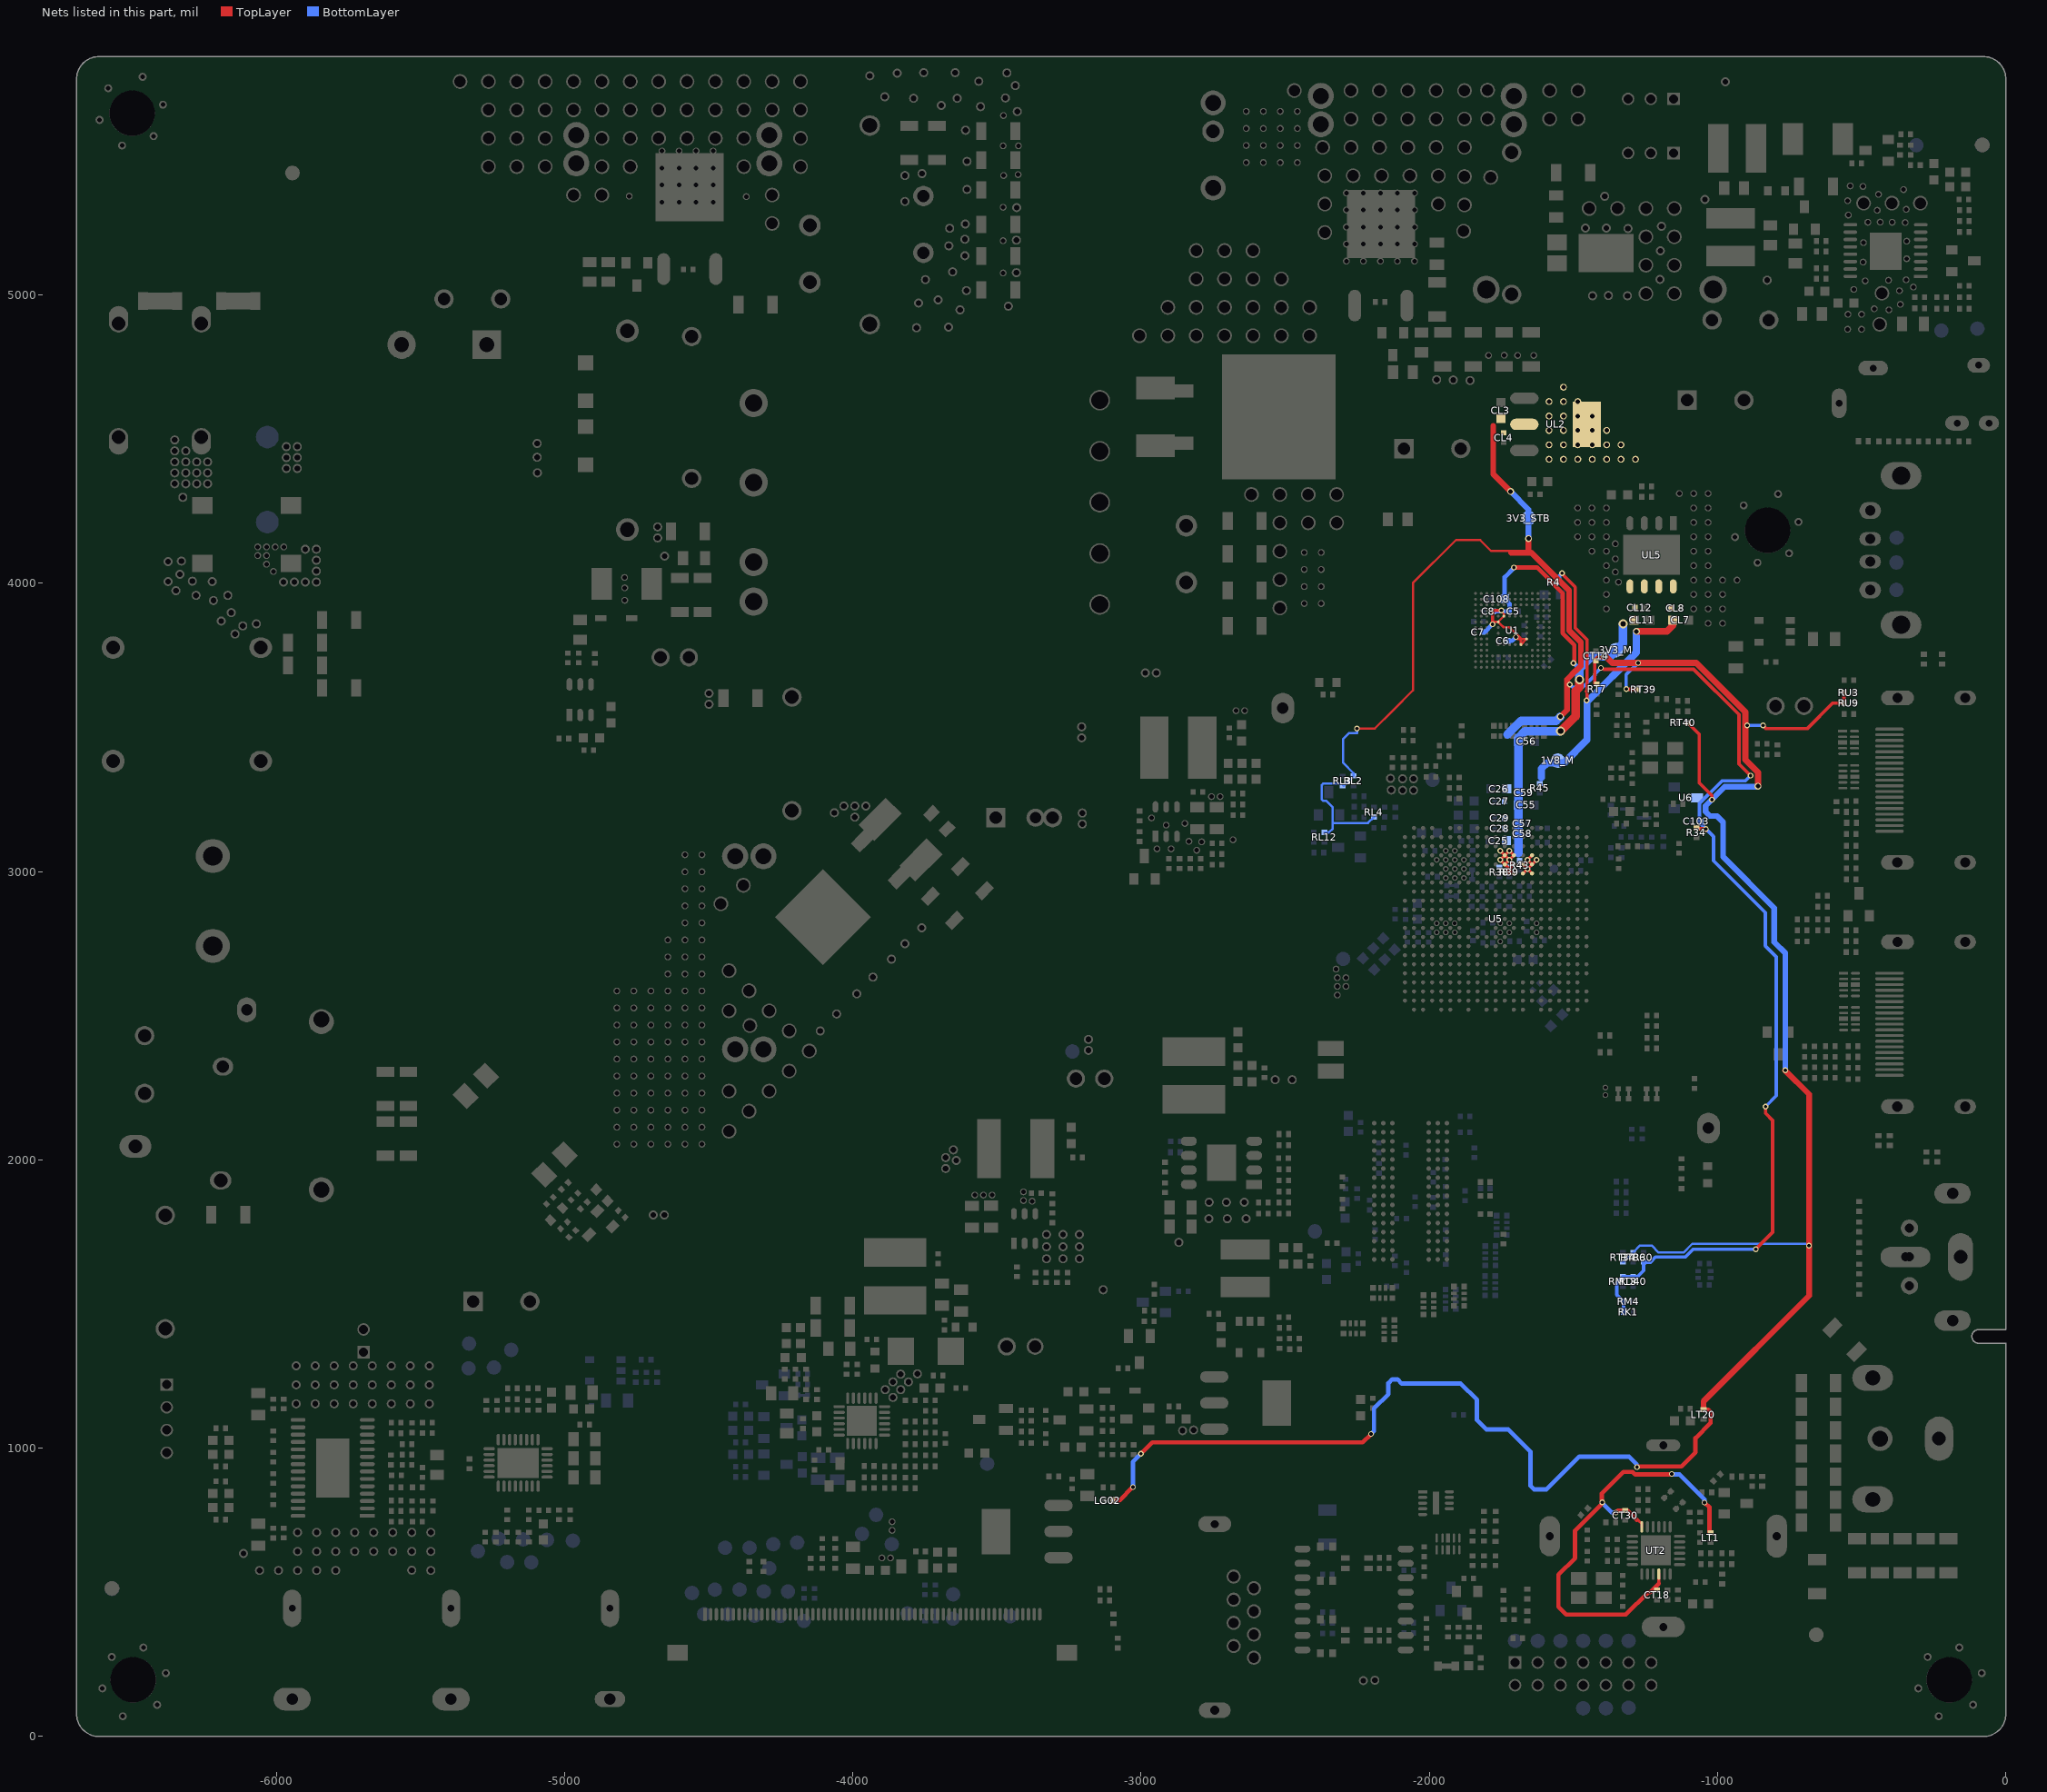
[diagram p0: the nets of this part, all layers, seen from the top]
# Altium PCB MISC84395.PcbDoc (part 8 of 26)
Units mil, origin at the board's own origin, x right, y up, seen from the top; angles counter-clockwise.
Board outline 6692.91 x 5826.77 mil, 2 copper layers (TopLayer, BottomLayer), stack 61.855 mil thick; 951 components, 565 nets, 4374 pads, 1804 vias.
Unrouted connection lines stored in the file: 1.

## Free pads (board coordinates)
  round 157.48 on Keep-Out: 0(-13188.98,196.85) 0(-6305.12,5435.04) 0(-196.85,5629.92) 1(-391.73,393.7)
  oval 196.85x157.48 on Keep-Out: 0(-12395.74,5629.92) 0(-990.09,196.85)
  round 47.24 on Bottom Solder: 0(-6402,5173)
  round 31.5 hole 19.68 paste-15.75 mask-15.75: VIA5(-6375,4006) VIA5(-6375,4075) VIA5(-6352,4345) VIA5(-6352,4383) VIA5(-6352,4421) VIA5(-6352,4459) VIA5(-6352,4497) VIA5(-6348,3974) VIA5(-6334,4031) VIA5(-6329,4077) VIA5(-6324,4298) VIA5(-6314,4345) VIA5(-6314,4383) VIA5(-6314,4421) VIA5(-6314,4459) VIA5(-6291,4007) VIA5(-6278,3958) VIA5(-6276,4345) VIA5(-6276,4383) VIA5(-6276,4421) VIA5(-6238,4345) VIA5(-6238,4383) VIA5(-6238,4421) VIA5(-6222,4006) VIA5(-6218,3940) VIA5(-6191,3869) VIA5(-6168,3958) VIA5(-6156,3898) VIA5(-6143,3824) VIA5(-6116,3852) VIA5(-6113.94,635) VIA5(-6069,3859) VIA5(-6057.94,576) VIA5(-5991.94,576) VIA5(-5975,4004) VIA5(-5965,4398) VIA5(-5965,4436) VIA5(-5965,4474) VIA5(-5937,4004) VIA5(-5930.94,1286) VIA5(-5930.94,1220) VIA5(-5930.94,1154) VIA5(-5927,4398) VIA5(-5927,4436) VIA5(-5927,4474) VIA5(-5925.94,576) VIA5(-5925.94,642) VIA5(-5925.94,708) VIA5(-5899,4004) VIA5(-5899,4118) VIA5(-5864.94,1286) VIA5(-5864.94,1154) VIA5(-5864.94,1220) VIA5(-5861,4004) VIA5(-5861,4042) VIA5(-5861,4080) VIA5(-5861,4118) VIA5(-5859.94,576) VIA5(-5859.94,642) VIA5(-5859.94,708) VIA5(-5798.94,1286) VIA5(-5798.94,1220) VIA5(-5798.94,1154) VIA5(-5793.94,576) VIA5(-5793.94,642) VIA5(-5793.94,708) VIA5(-5732.94,1286) VIA5(-5732.94,1154) VIA5(-5732.94,1220) VIA5(-5727.94,642) VIA5(-5727.94,708) VIA5(-5666.95,1286) VIA5(-5666.94,1154) VIA5(-5666.94,1220) VIA5(-5661.94,642) VIA5(-5661.94,708) VIA5(-5600.95,1286) VIA5(-5600.95,1154) VIA5(-5600.95,1220) VIA5(-5595.94,642) VIA5(-5595.94,708) VIA5(-5534.95,1286) VIA5(-5534.95,1154) VIA5(-5534.95,1220) VIA5(-5530,577) VIA5(-5529.94,642) VIA5(-5529.94,708) VIA5(-5468.95,1286) VIA5(-5468.95,1154) VIA5(-5468.95,1220) VIA5(-5463.94,576) VIA5(-5463.94,642) VIA5(-5463.94,708) VIA5(-5095.08,4437) VIA5(-5095.08,4485) VIA5(-5094,4383) VIA5(-4692,1809) VIA5(-4677,4157.3) VIA5(-4677,4195.3) VIA5(-4654,1809) VIA5(-4653,4094.3) VIA5(-4499,3580) VIA5(-4499,3618) VIA5(-4113,2447) VIA5(-4064,3204) VIA5(-4056,2506) VIA5(-4031,3227) VIA5(-3993,3189) VIA5(-3993,3227) VIA5(-3986,2576) VIA5(-3955,3227) VIA5(-3941,5760) VIA5(-3930,2634) VIA5(-3889,5687) VIA5(-3887.61,1203.13) VIA5(-3866,2696) VIA5(-3860.74,1176.26) VIA5(-3860.74,1230) VIA5(-3846,5769) VIA5(-3833.87,1203.13) VIA5(-3833.87,1256.87) VIA5(-3819,2750) VIA5(-3819,5324) VIA5(-3819,5414) VIA5(-3807,1230) VIA5(-3789,5682) VIA5(-3779,4886) VIA5(-3776,1258) VIA5(-3772,4972) VIA5(-3761,2805) VIA5(-3760,5421) VIA5(-3754,5771) VIA5(-3748,5053) VIA5(-3704,4983) VIA5(-3693,5657) VIA5(-3677.87,1970.13) VIA5(-3677.87,2008.13) VIA5(-3668,4888) VIA5(-3667,5170) VIA5(-3664,5231) VIA5(-3654,5080) VIA5(-3651,2035) VIA5(-3645,5771) VIA5(-3641.13,1998.13) VIA5(-3638,5682) VIA5(-3628,4948) VIA5(-3611,5136) VIA5(-3611,5193) VIA5(-3610,5246) VIA5(-3609,5571) VIA5(-3606,5015) VIA5(-3604,5366) VIA5(-3604,5463) VIA5(-3563,5741) VIA5(-3557,5653) VIA5(-3470.56,5683) VIA5(-3465.56,5770) VIA5(-3460.56,4961) VIA5(-3436.56,5726) VIA5(-3432.56,5077) VIA5(-3432.56,5190) VIA5(-3431.56,5303) VIA5(-3429.56,5636) VIA5(-3328,1657) VIA5(-3328,1699) VIA5(-3328,1741) VIA5(-3271,1657) VIA5(-3271,1699) VIA5(-3271,1741) VIA5(-3214,1657) VIA5(-3214,1699) VIA5(-3214,1741) VIA5(-3206,3464) VIA5(-3206,3502) VIA5(-3204,3165) VIA5(-3204,3203) VIA5(-3182.5,2380) VIA5(-3182.5,2418) VIA5(-3131.42,1549.58) VIA5(-2985.23,3688.77) VIA5(-2947.23,3688.77) VIA5(-2869,1714) VIA5(-2856,1061) VIA5(-2818,1063) VIA5(-2765,1796) VIA5(-2764,1853) VIA5(-2704,1853) VIA5(-2701,1796) VIA5(-2642,1853) VIA5(-2636,1796) VIA5(-2535,2278) VIA5(-2476,2278) VIA5(-2228.87,194.13) VIA5(-2189,195) VIA5(-2135,3323) VIA5(-2132,3283) VIA5(-2093,3282) VIA5(-2093,3322) VIA5(-2055,3282) VIA5(-2055,3322) VIA5(-1975,4706) VIA5(-1917,4705) VIA5(-1859,4703) VIA5(-1458.89,5232) VIA5(-1433.89,4997) VIA5(-1391.89,5342) VIA5(-1385.89,5232) VIA5(-1378.89,4998) VIA5(-1312.89,4997) VIA5(-1310.89,5230) VIA5(-1199.89,5054) VIA5(-1198.89,5153) VIA5(-1194.89,5238) VIA5(-1044,5331) VIA5(-973,5739) VIA5(-828,5051)
  round 23.62 hole 15.75 paste-15.75 mask-15.75: VIA5(-6064,4096) VIA5(-6064,4126) VIA5(-6034,4066) VIA5(-6034,4096) VIA5(-6034,4126) VIA5(-6010,4041) VIA5(-6004,4126) VIA5(-5974,4126) VIA5(-4818.66,2054.38) VIA5(-4818.66,2113.43) VIA5(-4818.66,2172.49) VIA5(-4818.66,2231.54) VIA5(-4818.66,2290.6) VIA5(-4818.66,2349.65) VIA5(-4818.66,2408.71) VIA5(-4818.66,2467.76) VIA5(-4818.66,2526.82) VIA5(-4818.66,2585.87) VIA5(-4792,4020) VIA5(-4791,3941) VIA5(-4791,3984) VIA5(-4775.66,5342.71) VIA5(-4759.6,2054.38) VIA5(-4759.6,2113.43) VIA5(-4759.6,2172.49) VIA5(-4759.6,2231.54) VIA5(-4759.6,2290.6) VIA5(-4759.6,2349.65) VIA5(-4759.6,2408.71) VIA5(-4759.6,2467.76) VIA5(-4759.6,2526.82) VIA5(-4759.6,2585.87) VIA5(-4700.55,2054.38) VIA5(-4700.55,2113.43) VIA5(-4700.55,2172.49) VIA5(-4700.55,2231.54) VIA5(-4700.55,2290.6) VIA5(-4700.55,2349.65) VIA5(-4700.55,2408.71) VIA5(-4700.55,2467.76) VIA5(-4700.55,2526.82) VIA5(-4700.55,2585.87) VIA5(-4661.66,5321.71) VIA5(-4661.66,5380.76) VIA5(-4661.66,5439.82) VIA5(-4661.66,5498.87) VIA5(-4641.49,2054.38) VIA5(-4641.49,2113.43) VIA5(-4641.49,2172.49) VIA5(-4641.49,2231.54) VIA5(-4641.49,2290.6) VIA5(-4641.49,2349.65) VIA5(-4641.49,2408.71) VIA5(-4641.49,2467.76) VIA5(-4641.49,2526.82) VIA5(-4641.49,2585.87) VIA5(-4641.49,2644.93) VIA5(-4641.49,2703.99) VIA5(-4641.49,2763.04) VIA5(-4602.6,5321.71) VIA5(-4602.6,5380.76) VIA5(-4602.6,5439.82) VIA5(-4602.6,5498.87) VIA5(-4582.44,2054.38) VIA5(-4582.44,2113.43) VIA5(-4582.44,2172.49) VIA5(-4582.44,2231.54) VIA5(-4582.44,2290.6) VIA5(-4582.44,2349.65) VIA5(-4582.44,2408.71) VIA5(-4582.44,2467.76) VIA5(-4582.44,2526.82) VIA5(-4582.44,2585.87) VIA5(-4582.44,2644.93) VIA5(-4582.44,2703.99) VIA5(-4582.44,2763.04) VIA5(-4582.44,2822.1) VIA5(-4582.44,2881.15) VIA5(-4582.44,2940.21) VIA5(-4582.44,2999.26) VIA5(-4582.44,3058.32) VIA5(-4543.55,5321.71) VIA5(-4543.55,5380.76) VIA5(-4543.55,5439.82) VIA5(-4543.55,5498.87) VIA5(-4523.38,2054.38) VIA5(-4523.38,2113.43) VIA5(-4523.38,2172.49) VIA5(-4523.38,2231.54) VIA5(-4523.38,2290.6) VIA5(-4523.38,2349.65) VIA5(-4523.38,2408.71) VIA5(-4523.38,2467.76) VIA5(-4523.38,2526.82) VIA5(-4523.38,2585.87) VIA5(-4523.38,2644.93) VIA5(-4523.38,2703.99) VIA5(-4523.38,2763.04) VIA5(-4523.38,2822.1) VIA5(-4523.38,2881.15) VIA5(-4523.38,2940.21) VIA5(-4523.38,2999.26) VIA5(-4523.38,3058.32) VIA5(-4484.49,5321.71) VIA5(-4484.49,5380.76) VIA5(-4484.49,5439.82) VIA5(-4484.49,5498.87) VIA5(-4369.66,5340.71) VIA5(-3899,619.5) VIA5(-3869,619.5) VIA5(-3864,715) VIA5(-3864,745) VIA5(-3577,1878) VIA5(-3547,1878) VIA5(-3517,1878) VIA5(-3478.56,5076) VIA5(-3478.56,5188) VIA5(-3478.56,5304) VIA5(-3478.56,5517) VIA5(-3477.56,5622) VIA5(-3476.56,5414) VIA5(-3426.56,5417) VIA5(-3425.56,5517) VIA5(-3408,1859) VIA5(-3408,1889) VIA5(-3378,1857) VIA5(-2964,3186) VIA5(-2944.83,3078.43) VIA5(-2913,3161) VIA5(-2895.85,3078.43) VIA5(-2848,3166.69) VIA5(-2834,3105) VIA5(-2807,3074) VIA5(-2790,3103) VIA5(-2756,3260) VIA5(-2726,3260) VIA5(-2681,3110) VIA5(-2671,3558) VIA5(-2641,3558) VIA5(-2635.01,5459.37) VIA5(-2635.01,5518.43) VIA5(-2635.01,5577.48) VIA5(-2635.01,5636.54) VIA5(-2575.95,5459.37) VIA5(-2575.95,5518.43) VIA5(-2575.95,5577.48) VIA5(-2575.95,5636.54) VIA5(-2516.9,5459.37) VIA5(-2516.9,5518.43) VIA5(-2516.9,5577.48) VIA5(-2516.9,5636.54) VIA5(-2457.84,5459.37) VIA5(-2457.84,5518.43) VIA5(-2457.84,5577.48) VIA5(-2457.84,5636.54) VIA5(-2434.06,3929.43) VIA5(-2434.06,3988.48) VIA5(-2434.06,4047.54) VIA5(-2434.06,4106.59) VIA5(-2375.01,3929.43) VIA5(-2375.01,3988.48) VIA5(-2375.01,4047.54) VIA5(-2375.01,4106.59) VIA5(-2323.65,2661.74) VIA5(-2319.65,2571.74) VIA5(-2319.65,2601.74) VIA5(-2319.65,2631.74) VIA5(-2289.65,2601.74) VIA5(-2289.65,2631.74) VIA5(-2288.06,5117.37) VIA5(-2288.06,5176.43) VIA5(-2288.06,5235.48) VIA5(-2288.06,5294.54) VIA5(-2288.06,5353.59) VIA5(-2229.01,5117.37) VIA5(-2229.01,5176.43) VIA5(-2229.01,5235.48) VIA5(-2229.01,5294.54) VIA5(-2229.01,5353.59) VIA5(-2169.95,5117.37) VIA5(-2169.95,5176.43) VIA5(-2169.95,5235.48) VIA5(-2169.95,5294.54) VIA5(-2169.95,5353.59) VIA5(-2110.9,5117.37) VIA5(-2110.9,5176.43) VIA5(-2110.9,5235.48) VIA5(-2110.9,5294.54) VIA5(-2110.9,5353.59) VIA5(-2051.84,5117.37) VIA5(-2051.84,5176.43) VIA5(-2051.84,5235.48) VIA5(-2051.84,5294.54) VIA5(-2051.84,5353.59) VIA5(-1795,4790) VIA5(-1740,4791) VIA5(-1694,4790) VIA5(-1638,4790) VIA5(-1585,4430) VIA5(-1585,4480) VIA5(-1585,4530) VIA5(-1585,4580) VIA5(-1585,4630) VIA5(-1535,4430) VIA5(-1535,4480) VIA5(-1535,4530) VIA5(-1535,4580) VIA5(-1535,4630) VIA5(-1535,4680) VIA5(-1486,4161) VIA5(-1486,4211) VIA5(-1486,4261) VIA5(-1485,4430) VIA5(-1485,4480) VIA5(-1485,4530) VIA5(-1485,4580) VIA5(-1485,4630) VIA5(-1436,4111) VIA5(-1436,4161) VIA5(-1436,4211) VIA5(-1436,4261) VIA5(-1435,4430) VIA5(-1435,4480) VIA5(-1435,4530) VIA5(-1435,4580) VIA5(-1386,3911) VIA5(-1386,3961) VIA5(-1386,4011) VIA5(-1386,4061) VIA5(-1386,4111) VIA5(-1386,4161) VIA5(-1386,4211) VIA5(-1386,4261) VIA5(-1385,4430) VIA5(-1385,4480) VIA5(-1385,4530) VIA5(-1355,4039) VIA5(-1355,4084.5) VIA5(-1355,4137) VIA5(-1344,4004) VIA5(-1335,4430) VIA5(-1335,4480) VIA5(-1285,4430) VIA5(-1133.04,4311) VIA5(-1083.04,4061) VIA5(-1083.04,4111) VIA5(-1083.04,4161) VIA5(-1083.04,4211) VIA5(-1083.04,4261) VIA5(-1083.04,4311) VIA5(-1083.04,3911) VIA5(-1083.04,3961) VIA5(-1083.04,4011) VIA5(-1033.04,3861) VIA5(-1033.04,3911) VIA5(-1033.04,3961) VIA5(-1033.04,4011) VIA5(-1033.04,4061) VIA5(-1033.04,4111) VIA5(-1033.04,4161) VIA5(-1033.04,4211) VIA5(-1033.04,4261) VIA5(-1033.04,4311) VIA5(-983.04,3911) VIA5(-983.04,4011) VIA5(-983.04,3861) VIA5(-983.04,3961) VIA5(-933.04,4011) VIA5(-549.19,5326.87) VIA5(-549,4881) VIA5(-548,4933) VIA5(-546.69,5276.87) VIA5(-540,5378) VIA5(-528,5019) VIA5(-501,4881) VIA5(-501,4933) VIA5(-496,5376) VIA5(-495.19,5113.87) VIA5(-494.19,5181.37) VIA5(-488.19,5048.37) VIA5(-479.19,5251.87) VIA5(-457,4952) VIA5(-446.19,5293.37) VIA5(-442,5349) VIA5(-436.19,5252.37) VIA5(-407.19,5050.87) VIA5(-406,4948) VIA5(-394.69,5251.79) VIA5(-369.19,5014.37) VIA5(-366.19,4967.37) VIA5(-355,5365) VIA5(-349.69,5250.87) VIA5(-346.19,5052.37) VIA5(-345.69,5296.87) VIA5(-344.19,5125.37) VIA5(-344.19,5186.37) VIA5(-321,5027)
  round 51.18 hole 39.37 paste-25.59 mask-2: VIA5(-5362.49,5740.1) VIA5(-5264.06,5444.82) VIA5(-5264.06,5543.25) VIA5(-5264.06,5641.67) VIA5(-5264.06,5740.1) VIA5(-5165.64,5444.82) VIA5(-5165.64,5543.25) VIA5(-5165.64,5641.67) VIA5(-5165.64,5740.1) VIA5(-5067.21,5444.82) VIA5(-5067.21,5543.25) VIA5(-5067.21,5641.67) VIA5(-5067.21,5740.1) VIA5(-4968.79,5346.4) VIA5(-4968.79,5641.67) VIA5(-4968.79,5740.1) VIA5(-4870.36,5346.4) VIA5(-4870.36,5444.82) VIA5(-4870.36,5543.25) VIA5(-4870.36,5641.67) VIA5(-4870.36,5740.1) VIA5(-4771.94,5444.82) VIA5(-4771.94,5543.25) VIA5(-4771.94,5641.67) VIA5(-4771.94,5740.1) VIA5(-4673.51,5543.25) VIA5(-4673.51,5641.67) VIA5(-4673.51,5740.1) VIA5(-4575.09,5543.25) VIA5(-4575.09,5641.67) VIA5(-4575.09,5740.1) VIA5(-4476.66,5543.25) VIA5(-4476.66,5641.67) VIA5(-4476.66,5740.1) VIA5(-4457.6,2888.4) VIA5(-4429.38,2517.02) VIA5(-4429.38,2656.21) VIA5(-4429.37,2099.43) VIA5(-4429.37,2238.63) VIA5(-4379.6,2952.4) VIA5(-4378.24,5444.82) VIA5(-4378.24,5543.25) VIA5(-4378.24,5641.67) VIA5(-4378.24,5740.1) VIA5(-4359.78,2586.61) VIA5(-4359.78,2169.03) VIA5(-4357,2466) VIA5(-4290.18,2517.02) VIA5(-4290.18,2238.63) VIA5(-4279.81,5247.97) VIA5(-4279.81,5346.4) VIA5(-4279.81,5641.67) VIA5(-4279.81,5740.1) VIA5(-4220.58,2447.42) VIA5(-4220.58,2308.22) VIA5(-4181.39,5444.82) VIA5(-4181.39,5543.25) VIA5(-4181.39,5641.67) VIA5(-4181.39,5740.1) VIA5(-4150.99,2377.82) VIA5(-3005.8,4858.41) VIA5(-2907.38,4858.41) VIA5(-2907.38,4956.83) VIA5(-2808.95,4858.41) VIA5(-2808.95,4956.83) VIA5(-2808.95,5055.26) VIA5(-2808.95,5153.68) VIA5(-2710.53,4858.41) VIA5(-2710.53,4956.83) VIA5(-2710.53,5055.26) VIA5(-2710.53,5153.68) VIA5(-2616.95,4307.83) VIA5(-2612.1,4858.41) VIA5(-2612.1,4956.83) VIA5(-2612.1,5055.26) VIA5(-2612.1,5153.68) VIA5(-2518.53,3914.13) VIA5(-2518.53,4012.56) VIA5(-2518.53,4110.98) VIA5(-2518.53,4209.41) VIA5(-2518.53,4307.83) VIA5(-2513.68,4858.41) VIA5(-2513.68,4956.83) VIA5(-2513.68,5055.26) VIA5(-2468.65,5708.68) VIA5(-2420.1,4209.41) VIA5(-2420.1,4307.83) VIA5(-2415.25,4858.41) VIA5(-2415.25,4956.83) VIA5(-2370.23,5511.83) VIA5(-2362.8,5216.56) VIA5(-2362.8,5314.98) VIA5(-2362.8,5413.41) VIA5(-2321.68,4209.41) VIA5(-2321.68,4307.83) VIA5(-2271.8,5511.83) VIA5(-2271.8,5610.26) VIA5(-2271.8,5708.68) VIA5(-2264.38,5413.41) VIA5(-2173.38,5511.83) VIA5(-2173.38,5610.26) VIA5(-2173.38,5708.68) VIA5(-2165.95,5413.41) VIA5(-2074.95,5511.83) VIA5(-2074.95,5610.26) VIA5(-2074.95,5708.68) VIA5(-2067.53,5413.41) VIA5(-1976.53,5511.83) VIA5(-1976.53,5610.26) VIA5(-1976.53,5708.68) VIA5(-1969.1,5314.98) VIA5(-1969.1,5413.41) VIA5(-1881,5221.09) VIA5(-1878.1,5312.09) VIA5(-1878.1,5410.51) VIA5(-1878.1,5511.83) VIA5(-1878.1,5610.26) VIA5(-1878.1,5708.68) VIA5(-1798.3,5709.9) VIA5(-1797.8,5610.8) VIA5(-1787.1,5407.61) VIA5(-1582.83,5708.68) VIA5(-1582.83,5610.26) VIA5(-1484.4,5708.68) VIA5(-1484.4,5610.26) VIA5(-1445.73,5299.72) VIA5(-1347.3,5299.72) VIA5(-1248.88,5004.44) VIA5(-1248.88,5102.87) VIA5(-1248.88,5201.29) VIA5(-1248.88,5299.72) VIA5(-1150.45,5004.44) VIA5(-1150.45,5102.87) VIA5(-1150.45,5201.29) VIA5(-1150.45,5299.72) VIA5(-493.61,5318.37) VIA5(-438,4898) VIA5(-430.19,5005.87) VIA5(-395.19,5318.37) VIA5(-296.76,5318.37)
  round 19.68 hole 11.81: VIA5(-1974.69,2788.84) VIA5(-1974.69,2820.34) VIA5(-1974.69,3040.81) VIA5(-1943.2,2788.84) VIA5(-1943.2,2820.34) VIA5(-1943.2,2977.82) VIA5(-1943.2,3009.31) VIA5(-1943.2,3040.81) VIA5(-1943.2,3072.3) VIA5(-1912.18,2820.33) VIA5(-1911.7,2788.84) VIA5(-1911.7,3009.31) VIA5(-1911.7,3040.81) VIA5(-1911.7,3072.3) VIA5(-1911.7,2977.82) VIA5(-1880.2,2977.82) VIA5(-1880.2,3009.31) VIA5(-1880.2,3040.81) VIA5(-1754.22,2757.34) VIA5(-1754.22,2788.84) VIA5(-1754.22,2820.34) VIA5(-1754.22,3040.81) VIA5(-1754.22,3072.3) VIA5(-1722.72,2788.84) VIA5(-1722.72,2820.34) VIA5(-1722.72,3040.81) VIA5(-1722.72,3072.3) VIA5(-1659.73,3009.31) VIA5(-1659.73,3040.81) VIA5(-1628.24,2788.84) VIA5(-1628.24,2820.34) VIA5(-1628.24,3040.81)
  round 19.68 hole 11.81 paste-15.75 mask-15.75: VIA5(-1389.65,2224.74) VIA5(-1389.65,2250.74)

## Via types
v1: diameter 19.68, hole 11.81, TopLayer to BottomLayer, tented both sides, 1262 vias
v2: diameter 23.62, hole 15.75, TopLayer to BottomLayer, tented both sides, 524 vias
v3: diameter 31.5, hole 19.68, TopLayer to BottomLayer, tented both sides, 11 vias
v4: diameter 24, hole 16, TopLayer to BottomLayer, tented both sides, 6 vias
v5: diameter 19, hole 11.81, TopLayer to BottomLayer, tented both sides, 1 vias

## Nets (pads, with @x,y where several pads share a name; then routed paths per layer and width w, separated by ;. In a path a pad name is that pad's centre, name@x,y a point inside that pad or via, vN(x,y) a via of type N, cw(c..) or ccw(c..) an arc to the next point about the centre after c; other vN are vias at no path point)
1.8VRF: CT18.1 CT30.2 LT1.1 UT2.12 UT2.22 | length 1611.4
  TopLayer w10: -1277.61,751.86 -1263.1,737.35 UT2.12@-1263.1,727.36 UT2.12@-1263.46,727 ; -1204.05,533 UT2.22@-1204.05,563.58
  TopLayer w15: v1@-1401.82,816.77 -1401.82,843.36 -1327.18,918 -1295,918 -1286,909 v1@-1159.5,909 ; v1(-1400,812) -1400,809 -1401.82,807.18 -1401.82,806.82 -1494.47,714.18 -1494.47,619.21 -1552,561.68 -1552,449.98 -1525.02,423 -1318.6,423 -1240.96,500.64 -1234.29,500.64 -1204.05,530.88 ; v1(-1353,777) -1346.26,783.74 CT30.2@-1321,783.74 ; CT30.2@-1313.57,784.28 -1281.14,751.86 ; v1@-1044.18,811.43 -1028.28,795.54 -1028.28,710.73 LT1.1@-1024.28,706.73
  BottomLayer w15: v1(-1400,812) -1400,809 -1368,777 v1(-1353,777) ; v1@-1159.5,909 -1132,909 -1046.11,823.11 v1(-1046.11,811.43)
  other v1: -1159.5,911
1V8_M: 1V8_M.1 CL7.2 CL8.2 R4.1 R45.1 UL5.7 UL5.8 | length 1380.1
  TopLayer w12: v1(-1540,4035) -1540,4032.18 -1494.15,3986.33 -1494.15,3845.04 -1453.21,3804.1 -1453.21,3661 ; v1(-1455,3594) -1453.21,3595.79 -1453.21,3661 ; -1455,3625 -1453.21,3626.79 -1453.21,3661
  TopLayer w24: v2(-1281.83,3833.02) -1176.2,3833.02 -1155.83,3853.4 CL7.2@-1155.83,3871.83
  BottomLayer w12: R4.1@-1548.46,4003 -1548.46,4026.54 v1(-1540,4035)
  BottomLayer w25: -1611.37,3326.41 -1611.37,3357.08 -1591.21,3377.23 -1532.77,3377.23 -1453,3457 -1453,3588.83 -1281.83,3760 v2@-1281.83,3833
3V3_M: 3V3_M.1 C5.2 C6.2 C7.2 C8.2 C55.2 C56.2 C57.2 C58.2 C59.2 C108.2 CL11.1 CL12.1 CT14.1 LG02.2 LT20.1 pad.VIA5@-1628.24,3040.81 pad.VIA5@-1659.73,3009.31 pad.VIA5@-1659.73,3040.81 R43.1 RT7.1 RT34.2 RT36.2 RT39.2 RT40.2 RU3.2 RU9.2 U1.E6 U1.F5 U1.J10 U1.K9 U5.T7 U5.T8 U5.U7 U5.U8 U5.V7 UL5.5 UL5.6 | length 10428.2
  TopLayer w7: U1.J10@-1761.08,3866.08 U1.K9@-1741.39,3885.77 -1741.39,3893.53 v1@-1750.21,3902.34
  TopLayer w8: v1(-1780.76,3857.82) -1772.5,3866.08 U1.J10@-1761.08,3866.08 -1745.18,3850.19 -1742.15,3847.16 -1721.32,3847.16 -1682.34,3808.18 -1682.34,3807.03 ; v1(-1699.71,3813.34) -1693.39,3807.03 -1682.34,3807.03 ; -1682.34,3807.03 U1.E6@-1682.34,3787.34 U1.F5@-1662.65,3807.03 -1682.34,3807.03
  TopLayer w10: U5.T8@-1675.48,2993.56 pad.VIA5@-1659.73,3009.31 ; U5.T7@-1643.98,2993.56 pad.VIA5@-1659.73,3009.31 ; U5.V7@-1643.98,3056.56 pad.VIA5@-1659.73,3040.81 ; pad.VIA5@-1628.24,3040.81 U5.U7@-1643.98,3025.06 ; pad.VIA5@-1659.73,3009.31 U5.U8@-1675.48,3025.06 pad.VIA5@-1659.73,3040.81 ; pad.VIA5@-1659.73,3009.31 U5.U7@-1643.98,3025.06 ; pad.VIA5@-1659.73,3040.81 U5.U7@-1643.98,3025.06
  TopLayer w12: v1(-1780.76,3857.82) -1780.76,3899.24 -1774.16,3905.84 v1(-1750.21,3905.84) ; RT7.1@-1424,3649.73 -1426.21,3651.94 -1426.21,3734 -1417.37,3742.84 v2@-1398,3742.84 ; v1@-1316.83,3632 RT39.2@-1274.57,3632 ; RT40.2@-1103.27,3516 -1064.15,3476.88 -1064.15,3308.4 -1020,3264.26 v1(-1020,3249) ; v1(-842.3,3506.8) -831.18,3495.67 -689.88,3495.67 -601.56,3584 RU9.2@-561.57,3584 RU3.2@-561.57,3621
  TopLayer w15: LG02.2@-3098.26,819 -3074.61,819 v1(-3028.45,865.16) ; v1(-3000.32,980.97) -2961.29,1020 -2231.36,1020 v1(-2202.2,1049.16) ; v1(-1707,4054.43) -1706.68,4054.74 -1678,4054.74 ; -1658.65,4054.74 -1678,4054.74 ; v1(-1500,3723) -1496.9,3726.1 -1496.9,3786.28 -1537.65,3827.02 -1537.65,3965.69 -1626.69,4054.74 -1678,4054.74 ; v1(-1280.09,934.69) -1277.75,937.03 -1125.99,937.03 -1076.9,986.12 -1076.9,1035 -1024.5,1087.4 -1024.5,1125.5 -1032.73,1133.73 LT20.1@-1049,1133.73
  TopLayer w20: LT20.1@-1049,1133.73 -1049,1163 -683,1529 v1(-683,1703) -683,2227.28 v1@-766.01,2310.29
  TopLayer w22: v2@-1387.88,3745.84 -1366.06,3724.02 v1(-1276,3724.02) -1074.35,3724.02 -904.15,3553.82 -904.15,3387.69 -860.16,3343.7 v2@-860.16,3295.84
  TopLayer w30: v3(-1544.65,3487.09) -1492.49,3539.25 -1492.49,3626.07 -1479.21,3639.35 v3(-1479.21,3666)
  BottomLayer w8: RT34.2@-1328.82,1645.52 -1326.3,1645.52 RT36.2@-1292.83,1678.99 -1268.82,1703 -1229.03,1703 -1204.32,1678.29 -1118.38,1678.29 -1087.51,1709.16 v1@-685.16,1709.16
  BottomLayer w12: v1@-1317.83,3633 -1317.83,3682.19 v1(-1276,3724.02) ; v1(-897.8,3506.8) v1(-842.3,3506.8) v1@-888.2,3506.8
  BottomLayer w15: v1(-3028.45,865.16) -3028.45,952.84 v1(-3000.32,980.97) ; v1(-2202.2,1049.16) -2192.34,1059.02 -2192.34,1137.73 -2142.21,1187.86 -2142.21,1225.65 -2129.12,1238.74 -2110.61,1238.74 -2096.22,1224.34 -1891.03,1224.34 -1834.91,1168.22 -1834.91,1097.73 -1802.68,1065.5 -1726.68,1065.5 -1649.5,988.32 -1649.5,870.07 -1636.93,857.5 -1593.21,857.5 -1479.9,970.81 -1307.49,970.81 -1280.09,943.41 v1(-1280.09,934.69) ; C7.2@-1813.91,3830.74 -1807.84,3830.74 v1(-1780.76,3857.82) ; C8.2@-1777.91,3902.74 -1721.38,3902.74 -1721.38,3928.28 C108.2@-1738.84,3945.74 -1738.84,4021.16 -1707,4053 v1(-1707,4054.43) ; C6.2@-1727.47,3799.84 -1713.21,3799.84 v1(-1699.71,3813.34) ; v1(-1500,3723) -1498.42,3723 -1479.21,3703.79
  BottomLayer w20: v2@-860.99,3293.84 -975.6,3293.84 -1041.84,3227.61 -1041.84,3207.03 -1027.28,3192.48 -1002.35,3192.48 -980.99,3171.12 -980.99,3051 -803.46,2873.46 -803.46,2755.26 -765.3,2717.1 v1(-765.3,2311)
  BottomLayer w30: -1691.23,3064.81 -1691.23,3464.16 -1668.29,3487.09 v3(-1544.65,3487.09) ; v3(-1479.21,3666) -1479.21,3703.79 -1437.16,3745.84 v2(-1393,3745.84) -1372.99,3745.84 -1327.83,3791 v3@-1327.83,3859
  other v1: -1316.83,3633
  other v2: -859.99,3295.84
  other v3: -1328,3859
3V3_STB: 3V3_STB.1 C25.2 C26.2 C27.2 C28.2 C29.2 C103.2 CL3.1 CL4.1 pad.VIA5@-1285,4430 pad.VIA5@-1335,4430 pad.VIA5@-1335,4480 pad.VIA5@-1385,4430 pad.VIA5@-1385,4480 pad.VIA5@-1385,4530 pad.VIA5@-1435,4430 pad.VIA5@-1435,4480 pad.VIA5@-1435,4530 pad.VIA5@-1435,4580 pad.VIA5@-1485,4430 pad.VIA5@-1485,4480 pad.VIA5@-1485,4530 pad.VIA5@-1485,4580 pad.VIA5@-1485,4630 pad.VIA5@-1535,4430 pad.VIA5@-1535,4480 pad.VIA5@-1535,4530 pad.VIA5@-1535,4580 pad.VIA5@-1535,4630 pad.VIA5@-1535,4680 pad.VIA5@-1585,4430 pad.VIA5@-1585,4480 pad.VIA5@-1585,4530 pad.VIA5@-1585,4580 pad.VIA5@-1585,4630 pad.VIA5@-1722.72,3040.81 pad.VIA5@-1722.72,3072.3 pad.VIA5@-1754.22,3040.81 pad.VIA5@-1754.22,3072.3 R30.1 R34.1 R38.1 R39.1 RD40.2 RK1.2 RL2.2 RL3.2 RL4.2 RL12.2 RM4.1 RM13.2 U5.T9 U5.T10 U5.U9 U5.U10 U5.V9 U5.V10 U6.3 UL2.2 UL2.4 | length 7020.6
  TopLayer w8: v1(-2251,3496) -2189.22,3496 -2127.37,3557.84 -2056.88,3628.34 -2056.88,4000.48 -1907.36,4150 -1824.03,4150 -1786.19,4112.16 -1722,4112.16
  TopLayer w10: pad.VIA5@-1754.22,3072.3 U5.V10@-1738.47,3056.56 ; U5.U10@-1738.47,3025.06 pad.VIA5@-1722.72,3040.81 ; U5.U10@-1738.47,3025.06 pad.VIA5@-1754.22,3040.81 U5.V10@-1738.47,3056.56 ; U5.U10@-1738.47,3025.06 -1722.72,3009.31 ; U5.V10@-1738.47,3056.56 pad.VIA5@-1722.72,3040.81 ; U5.V10@-1738.47,3056.56 pad.VIA5@-1722.72,3072.3 U5.V9@-1706.98,3056.56 pad.VIA5@-1722.72,3040.81 ; -1722.72,3009.31 U5.T10@-1738.47,2993.56 U5.T9@-1706.98,2993.56 -1722.72,3009.31 ; -1722.72,3009.31 U5.U9@-1706.98,3025.06 pad.VIA5@-1722.72,3040.81
  TopLayer w12: v1@-1518.49,3649 v1(-1513,3649) ; -1395.02,3702.02 -1083.47,3702.02 -926.15,3544.7 -926.15,3373.15 v1(-886,3333) ; R34.1@-1073,3151.73 -1070.11,3148.84 -1041.67,3148.84 v1(-1040.83,3148) v1@-1040.83,3143.78 ; v1(-867.68,1690.32) -809,1749 -809,2136.88 -834,2161.88 v1(-834,2185)
  TopLayer w20: -1778.5,4545.69 -1778.5,4378.39 v2(-1718,4318) ; -1716,4106.16 -1656,4106.16 ; v2(-1656,4155) -1656,4106.16 ; v2(-1546,3537) -1522.49,3560.51 -1522.49,3653 ; -1522.24,3653.24 -1522.49,3653 ; -1656,4106.16 -1646.29,4106.16 -1515.15,3975.01 -1515.15,3836.34 -1474.4,3795.6 -1474.4,3713.46 -1491.12,3696.75 -1491.94,3696.75 -1522.49,3666.2 -1522.49,3653
  BottomLayer w8: RL12.2@-2364,3135.73 -2348.27,3135.73 -2335.25,3148.75 -2335.25,3223.19 -2356.93,3244.88 -2368.48,3244.88 -2373.25,3249.65 -2373.25,3300.41 -2367.98,3305.69 -2305.62,3305.69 -2297.21,3297.27 RL2.2@-2263,3331.47 -2263,3341.3 -2298.84,3377.14 -2298.84,3460.02 -2279.02,3479.84 -2250.98,3479.84 v1@-2250.98,3495.98 ; -2332.56,3168.31 -2212.95,3168.31 RL4.2@-2192,3189.27
  BottomLayer w12: v1(-1513,3649) -1503.25,3639.25 -1468.13,3639.25 -1425.84,3681.54 ; -1425.84,3685.16 v1(-1405,3706) ; RM13.2@-1329,1592.73 RM13.2@-1328.77,1592.96 ; RM4.1@-1326.46,1509 -1349.62,1532.15 -1349.62,1574.95 -1329.57,1595 RM13.2@-1328.77,1595 -1278,1595 -1257,1616 R30.1@-1257,1645.38 -1233.32,1645.38 -1215.41,1663.29 -1112.17,1663.29 -1085.46,1690 v1@-867.68,1690 ; RK1.2@-1326.2,1472 RM4.1@-1326.2,1508.73 ; C103.2@-1062.84,3170 v1(-1040.83,3148) -1013.99,3121.16 -1013.99,3037.33 -834.46,2857.79 -834.46,2742.42 -796.3,2704.26 -796.3,2222.7 v1(-834,2185) ; C103.2@-1062.84,3174 -1062.84,3236.31 -984.3,3314.84 -904.16,3314.84 v1(-886,3333)
  BottomLayer w20: v2(-1718,4318) -1656,4256 3V3_STB.1@-1656,4226 v2(-1656,4155)
  BottomLayer w30: -1729.47,3475.42 -1682.14,3522.74 -1560.26,3522.74 v2(-1546,3537)